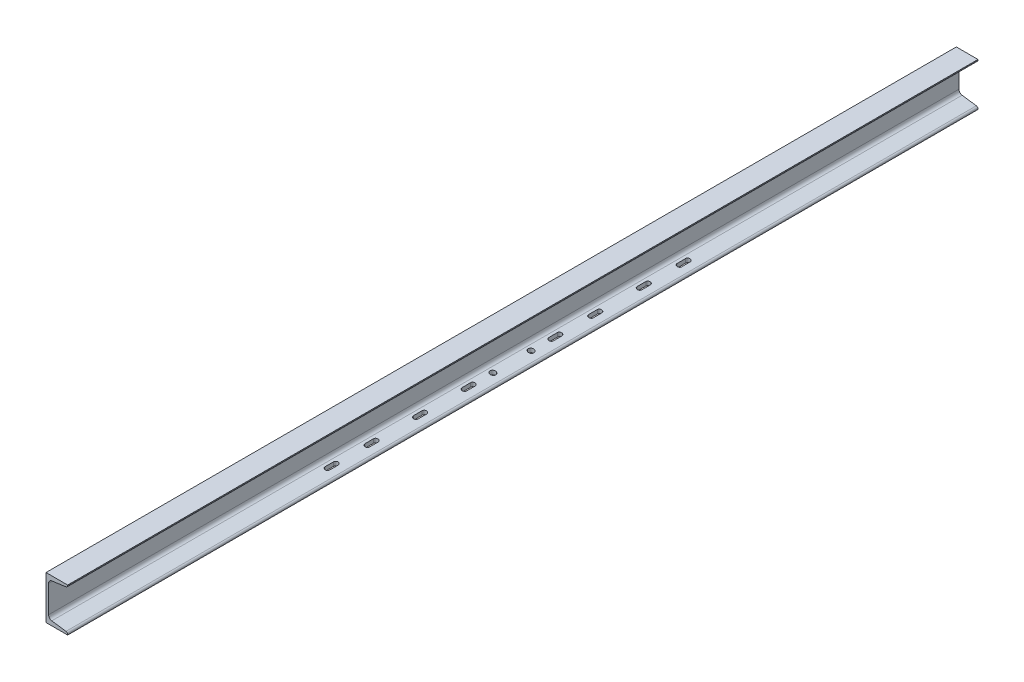
from build123d import *

# Parameters (mm, degrees)
EXTRUDE_1_DEPTH     = 2100
SKETCH_2_R          = 6.5
CUT_EXTRUDE_1_DEPTH = 2100
SKETCH_6_R          = 6.5
CUT_EXTRUDE_3_DEPTH = 10


with BuildPart() as part:
    # 草图1 → 凸台-拉伸1 (new body)
    with BuildSketch(Plane.XY):
        with BuildLine():
            Line((0, 0), (-50, 0))
            Line((-50, 0), (-50, -100))
            Line((-50, -100), (0, -100))
            Line((0, -100), (0, -98.925311188))
            ThreePointArc((0, -98.925311188), (-1.103806889, -95.973045557), (-3.873721046, -94.469104878))
            Line((-3.873721046, -94.469104878), (-36.682971358, -89.858065454))
            ThreePointArc((-36.682971358, -89.858065454), (-41.915031432, -87.017288616), (-44, -81.440786869))
            Line((-44, -81.440786869), (-44, -18.559213131))
            ThreePointArc((-44, -18.559213131), (-41.915031432, -12.982711384), (-36.682971358, -10.141934546))
            Line((-36.682971358, -10.141934546), (-3.873721046, -5.530895122))
            ThreePointArc((-3.873721046, -5.530895122), (-1.103806889, -4.026954443), (0, -1.074688812))
            Line((0, -1.074688812), (0, 0))
        make_face()
    extrude(amount=EXTRUDE_1_DEPTH)

    # 草图2 → 切除-拉伸1 (cut)
    with BuildSketch(Plane.ZY.offset(50)):
        with Locations(Location((59.6, -30, 0), (0, 0, 270))):
            Circle(SKETCH_2_R)
        with Locations(Location((183.4, -30, 0), (0, 0, 270))):
            Circle(SKETCH_2_R)
        with Locations(Location((307.2, -30, 0), (0, 0, 270))):
            Circle(SKETCH_2_R)
        with Locations(Location((431, -30, 0), (0, 0, 270))):
            Circle(SKETCH_2_R)
        with Locations(Location((554.8, -30, 0), (0, 0, 270))):
            Circle(SKETCH_2_R)
        with Locations(Location((678.6, -30, 0), (0, 0, 270))):
            Circle(SKETCH_2_R)
        with Locations(Location((802.4, -30, 0), (0, 0, 270))):
            Circle(SKETCH_2_R)
        with Locations(Location((926.2, -30, 0), (0, 0, 270))):
            Circle(SKETCH_2_R)
        with Locations(Location((1050, -30, 0), (0, 0, 270))):
            Circle(SKETCH_2_R)
        with Locations(Location((1173.8, -30, 0), (0, 0, 270))):
            Circle(SKETCH_2_R)
        with Locations(Location((1297.6, -30, 0), (0, 0, 270))):
            Circle(SKETCH_2_R)
        with Locations(Location((1421.4, -30, 0), (0, 0, 270))):
            Circle(SKETCH_2_R)
        with Locations(Location((1545.2, -30, 0), (0, 0, 270))):
            Circle(SKETCH_2_R)
        with Locations(Location((1669, -30, 0), (0, 0, 270))):
            Circle(SKETCH_2_R)
        with Locations(Location((1792.8, -30, 0), (0, 0, 270))):
            Circle(SKETCH_2_R)
        with Locations(Location((1916.6, -30, 0), (0, 0, 270))):
            Circle(SKETCH_2_R)
        with Locations(Location((2040.4, -30, 0), (0, 0, 270))):
            Circle(SKETCH_2_R)
    extrude(amount=-CUT_EXTRUDE_1_DEPTH, mode=Mode.SUBTRACT)

    # 草图6 → 切除-拉伸3 (cut)
    with BuildSketch(Plane.XZ.offset(100)):
        with Locations(Location((-25, 1006, 0), (0, 0, 270))):
            Circle(SKETCH_6_R)
        with Locations(Location((-25, 1094, 0), (0, 0, 270))):
            Circle(SKETCH_6_R)
        with BuildLine():
            Line((-30.25, 644), (-30.25, 664))
            ThreePointArc((-30.25, 664), (-25, 669.25), (-19.75, 664))
            Line((-19.75, 664), (-19.75, 644))
            ThreePointArc((-19.75, 644), (-25, 638.75), (-30.25, 644))
        make_face()
        with BuildLine():
            Line((-30.25, 736), (-30.25, 756))
            ThreePointArc((-30.25, 756), (-25, 761.25), (-19.75, 756))
            Line((-19.75, 756), (-19.75, 736))
            ThreePointArc((-19.75, 736), (-25, 730.75), (-30.25, 736))
        make_face()
        with BuildLine():
            Line((-19.75, 868), (-19.75, 848))
            ThreePointArc((-19.75, 848), (-25, 842.75), (-30.25, 848))
            Line((-30.25, 848), (-30.25, 868))
            ThreePointArc((-30.25, 868), (-25, 873.25), (-19.75, 868))
        make_face()
        with BuildLine():
            Line((-19.75, 960), (-19.75, 940))
            ThreePointArc((-19.75, 940), (-25, 934.75), (-30.25, 940))
            Line((-30.25, 940), (-30.25, 960))
            ThreePointArc((-30.25, 960), (-25, 965.25), (-19.75, 960))
        make_face()
        with BuildLine():
            Line((-19.75, 1272), (-19.75, 1252))
            ThreePointArc((-19.75, 1252), (-25, 1246.75), (-30.25, 1252))
            Line((-30.25, 1252), (-30.25, 1272))
            ThreePointArc((-30.25, 1272), (-25, 1277.25), (-19.75, 1272))
        make_face()
        with BuildLine():
            Line((-19.75, 1476), (-19.75, 1456))
            ThreePointArc((-19.75, 1456), (-25, 1450.75), (-30.25, 1456))
            Line((-30.25, 1456), (-30.25, 1476))
            ThreePointArc((-30.25, 1476), (-25, 1481.25), (-19.75, 1476))
        make_face()
        with BuildLine():
            Line((-19.75, 1384), (-19.75, 1364))
            ThreePointArc((-19.75, 1364), (-25, 1358.75), (-30.25, 1364))
            Line((-30.25, 1364), (-30.25, 1384))
            ThreePointArc((-30.25, 1384), (-25, 1389.25), (-19.75, 1384))
        make_face()
        with BuildLine():
            Line((-19.75, 1160), (-19.75, 1140))
            ThreePointArc((-19.75, 1140), (-25, 1134.75), (-30.25, 1140))
            Line((-30.25, 1140), (-30.25, 1160))
            ThreePointArc((-30.25, 1160), (-25, 1165.25), (-19.75, 1160))
        make_face()
    extrude(amount=-CUT_EXTRUDE_3_DEPTH, mode=Mode.SUBTRACT)


solid = part.part
